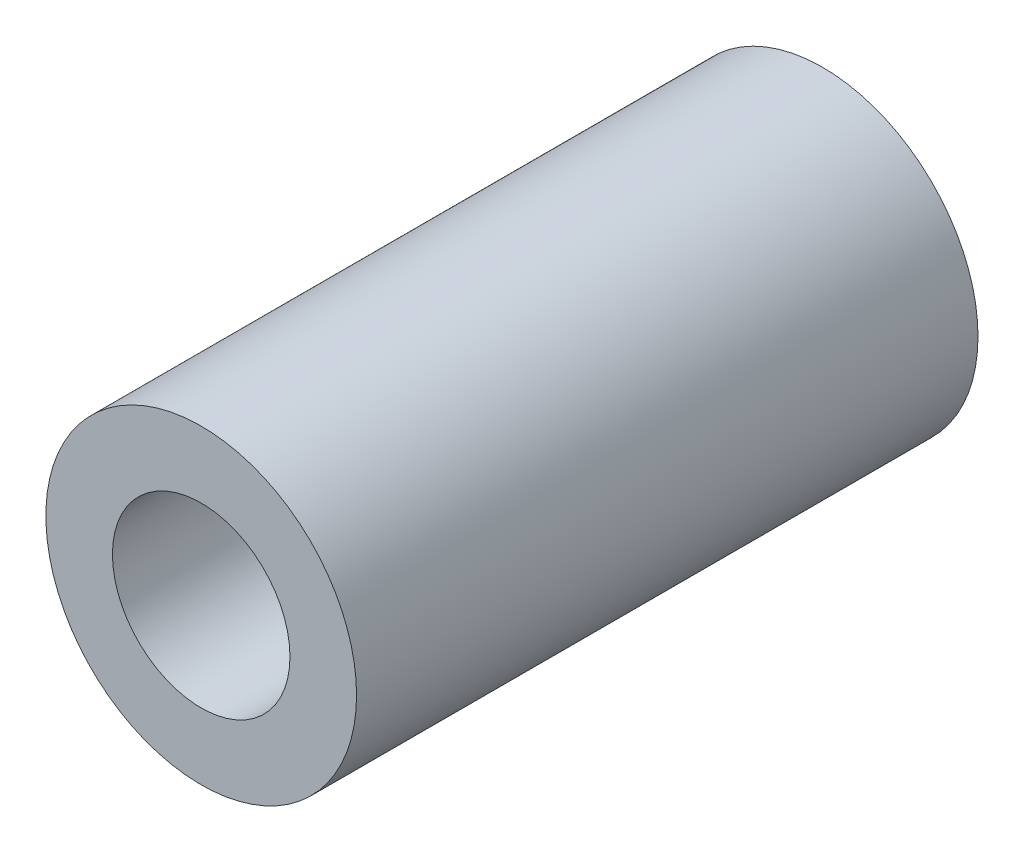
from build123d import *

# Parameters (mm, degrees)
SKETCH1_R           = 7
SKETCH1_R_2         = 4
BOSS_EXTRUDE1_DEPTH = 28


with BuildPart() as part:
    # Sketch1 → Boss-Extrude1 (new body)
    with BuildSketch(Plane.XY):
        Circle(SKETCH1_R)
        Circle(SKETCH1_R_2, mode=Mode.SUBTRACT)
    extrude(amount=-BOSS_EXTRUDE1_DEPTH)


solid = part.part
